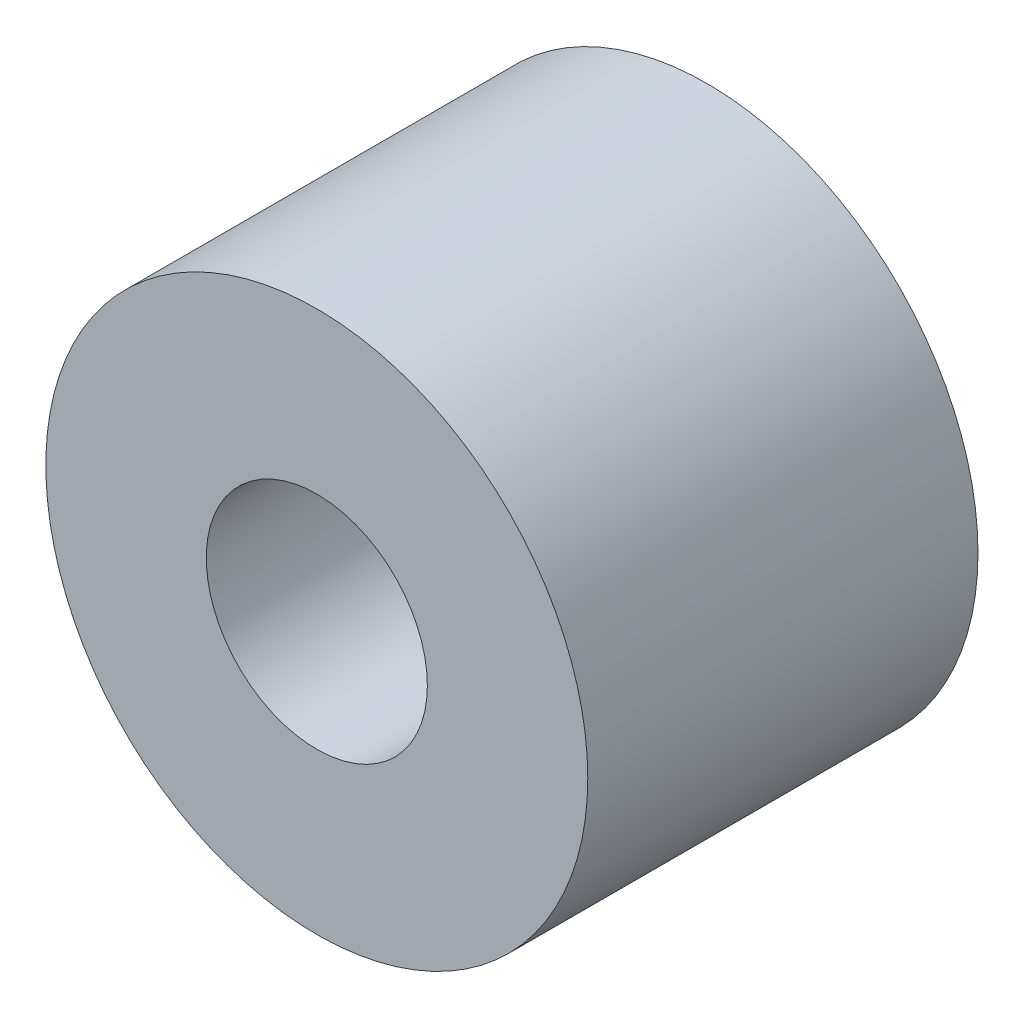
SolidWorks part; units mm, degrees
material "SS400B"
ref_plane "Front Plane" through (0, 0, 0) normal (0, 0, 1) x (1, 0, 0)
ref_plane "Top Plane" through (0, 0, 0) normal (0, 1, 0) x (1, 0, 0)
ref_plane "Right Plane" through (0, 0, 0) normal (1, 0, 0) x (0, 0, -1)
sketch "Sketch1" plane through (0, 0, 0) normal (0, 0, 1) x (1, 0, 0)
  circle A0 centre (0, 0) radius 12.5
  dimension "D1" = 25
extrude "Boss-Extrude1" add sketch "Sketch1" along normal blind 18
hole_wizard "M12 Tapped Hole1" positions "Sketch2" profile "Sketch3" tap size "M12" standard "GB"
sketch "Sketch2" plane through (0, 0, 18) normal (0, 0, 1) x (1, 0, 0)
  point P0 (0, 0)
sketch "Sketch3" plane through (0, 0, 18) normal (1, 0, 0) x (0, -1, 0)
  line L0 (0, 0) -> (0, 32.3144)
  line L1 (0, 32.3144) -> (5.1, 29.25)
  line L2 (5.1, 29.25) -> (5.1, 0)
  line L5 (5.1, 0) -> (0, 0)
  line L10 (0, 32.3144) -> (-5.1, 29.25) construction
  line L11 (0, -6.35) -> (0, 107.95) construction
  dimension "螺纹孔钻头直径" = 10.2
  dimension "螺纹孔钻头深度" = 29.25
  dimension "导头角度" = 118
cosmetic thread "Cosmetic-Thread1" parameters "D1"=24, "D2"=12
